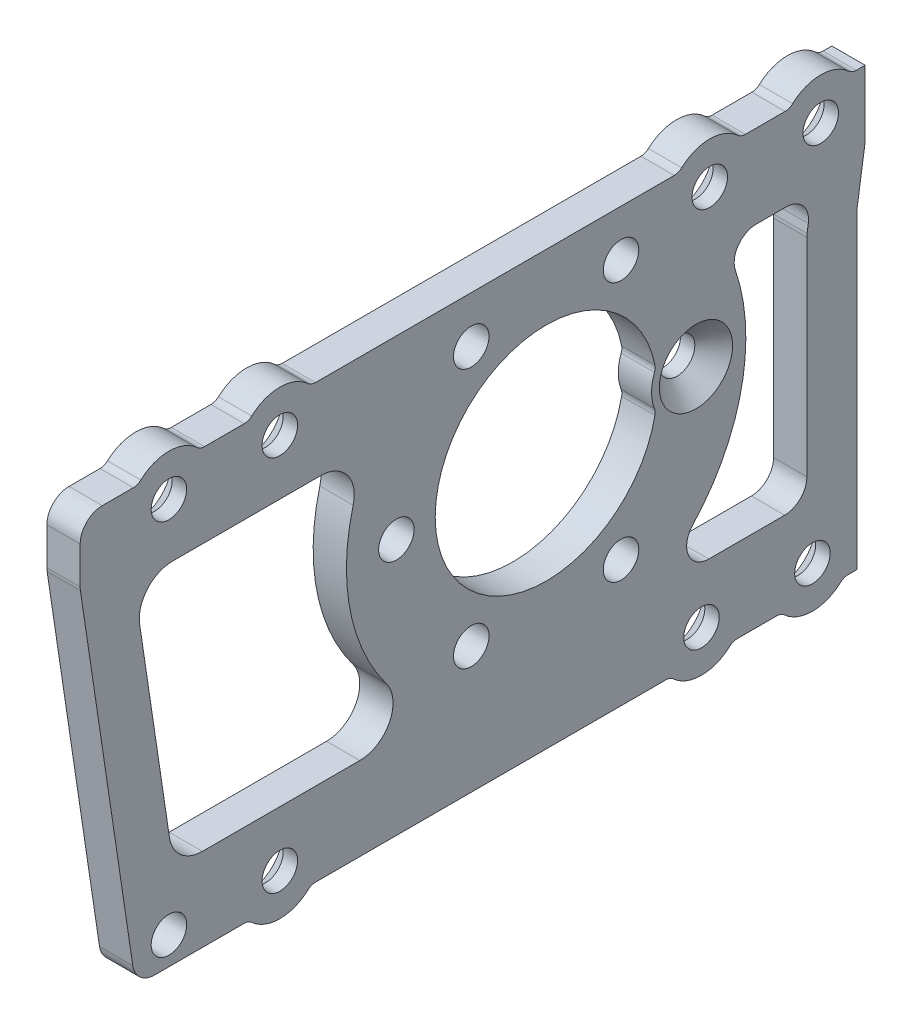
SolidWorks part; units mm, degrees
other "标注1"
sketch "草图13" plane through (3, 17.15, -28.75) normal (0.7677, 0.0888, -0.6346) x (-0.6353, 0.2347, -0.7357)
material "Thornel Mat VMA"
ref_plane "前视基准面" through (0, 0, 0) normal (0, 0, 1) x (1, 0, 0)
ref_plane "上视基准面" through (0, 0, 0) normal (0, 1, 0) x (1, 0, 0)
ref_plane "右视基准面" through (0, 0, 0) normal (1, 0, 0) x (0, 0, -1)
other "Configuration Table"
sketch "草图1" plane through (0, 0, 0) normal (1, 0, 0) x (0, 0, -1)
  line L0 (0, 0) -> (-13.5, 0) construction
  line L4 (0, 0) -> (0, -20.6) construction
  line L6 (28, 4.9) -> (28, -23.1)
  line L7 (28, -23.1) -> (-37, -23.1)
  line L9 (0, -20.6) -> (14, -20.6) construction
  line L10 (14, -20.6) -> (24, -20.6) construction
  line L11 (-51.8773, -23.6) -> (28, -23.6) construction
  line L12 (-55.4482, 16.4) -> (44.8007, 16.4) construction
  line L13 (28, 4.9) -> (28.75, 9.9)
  line L14 (28.75, 9.9) -> (28.75, 15.9)
  line L15 (28.75, 15.9) -> (-42, 15.9)
  line L16 (-42, 15.9) -> (-42, 10.4)
  line L17 (-37, -23.6) -> (-16, -23.6) construction
  line L18 (-37, -23.6) -> (-37, -17.6) construction
  line L19 (-37, -17.6) -> (-16, -17.6) construction
  line L20 (-16, -23.6) -> (-16, -17.6) construction
  line L21 (-42, 10.4) -> (-21, 10.4) construction
  line L22 (-42, 10.4) -> (-42, 16.4) construction
  line L23 (-42, 16.4) -> (-21, 16.4) construction
  line L24 (-21, 10.4) -> (-21, 16.4) construction
  line L25 (-42, 10.4) -> (-37, -23.1)
  circle A0 centre (0, 0) radius 13.5 construction
  circle A1 centre (-13.5, 0) radius 1.6
  circle A2 centre (-6.75, 11.6913) radius 1.6
  circle A3 centre (6.75, 11.6913) radius 1.6
  circle A4 centre (13.5, 0) radius 1.6
  circle A5 centre (6.75, -11.6913) radius 1.6
  circle A6 centre (-6.75, -11.6913) radius 1.6
  circle A7 centre (0, 0) radius 10
  circle A9 centre (14, -20.6) radius 1.6
  circle A10 centre (24, -20.6) radius 1.6
  circle A11 centre (24.75, 13.4) radius 1.6
  circle A12 centre (14.75, 13.4) radius 1.6
  circle A13 centre (0, 0) radius 28.5 construction
  circle A14 centre (-24, -20.6) radius 1.6 construction
  circle A15 centre (-34, -20.6) radius 1.6 construction
  circle A16 centre (-24, -20.6) radius 3 construction
  circle A17 centre (-24, -20.6) radius 1.6
  circle A18 centre (-34, -20.6) radius 1.6
  circle A19 centre (-34, 13.4) radius 1.6
  circle A20 centre (-24, 13.4) radius 1.6
  point P17 (0, 0)
  dimension "D1" = 27
  dimension "D2" = 3.2
  dimension "D4" = 20
  dimension "D5" = 3
  dimension "D10" = 3.2
  dimension "D12" = 3.2
  dimension "D16" = 3.2
  dimension "D17" = 3.2
  dimension "D18" = 10
  dimension "D19" = 8
  dimension "D23" = 57
  dimension "D26" = 3.2
  dimension "D27" = 3.2
  dimension "D28" = 24
  dimension "D29" = 3
  dimension "D30" = 10
  dimension "D32" = 6
  dimension "D33" = 3.2
  dimension "D34" = 3.2
  dimension "D6" = 23.1
  dimension "D7" = 28
  dimension "D8" = 14
  dimension "D9" = 20.6
  dimension "D11" = 10
  dimension "D13" = 4
  dimension "D14" = 0.5
  dimension "D15" = 40
  dimension "D20" = 6
  dimension "D21" = 1
  dimension "D22" = 4
  dimension "D24" = 21
  dimension "D25" = 6
  dimension "D31" = 3
  dimension "D35" = 3
  dimension "D36" = 3
  dimension "D37" = 10
  dimension "D38" = 3
  dimension "D39" = 6
  dimension "D40" = 3
  dimension "D41" = 8
  dimension "D3" = 6
extrude "凸台-拉伸1" add sketch "草图1" along normal blind 3
sketch "草图2" plane through (0, 0, 0) normal (-1, 0, 0) x (0, 0, 1)
  circle A0 centre (-24.75, 13.4) radius 1.6
  circle A1 centre (-24.75, 13.4) radius 3.75
  circle A2 centre (-14.75, 13.4) radius 1.6
  circle A3 centre (-14.75, 13.4) radius 3.75
  circle A4 centre (24, 13.4) radius 1.6
  circle A5 centre (24, 13.4) radius 3.75
  circle A6 centre (24, -20.6) radius 1.6
  circle A7 centre (24, -20.6) radius 3.75
  circle A8 centre (-24, -20.6) radius 1.6
  circle A9 centre (-14, -20.6) radius 1.6
  circle A10 centre (-24, -20.6) radius 3.75
  circle A11 centre (-14, -20.6) radius 3.75
  circle A14 centre (-13.5, 0) radius 1.6
  circle A15 centre (-13.5, 0) radius 4
  circle A16 centre (34, 13.4) radius 3.75
  circle A17 centre (34, 13.4) radius 1.6
  dimension "D1" = 7.5
  dimension "D2" = 3.2
  dimension "D3" = 3.2
  dimension "D4" = 7.5
  dimension "D5" = 3.2
  dimension "D6" = 7.5
  dimension "D7" = 3.2
  dimension "D8" = 7.5
  dimension "D9" = 3.2
  dimension "D10" = 3.2
  dimension "D11" = 7.5
  dimension "D12" = 7.5
  dimension "D13" = 8
  dimension "D14" = 3.2
  dimension "D15" = 7.5
  dimension "D16" = 3.2
extrude "凸台-拉伸2" add sketch "草图2" against normal up to surface (3 mm away) up to face at (3, 13.4, 32.4)
hole_wizard "M3 十字槽半沉头木螺钉的锥形沉头孔1" positions "草图16" profile "草图15" countersink size "M3" standard "GB"
sketch "草图16" plane through (0, 0, 0) normal (-1, 0, 0) x (0, 0, 1)
  point P0 (-24.75, 13.4)
  point P3 (-14.75, 13.4)
  point P6 (-24, -20.6)
  point P9 (-14, -20.6)
  point P12 (24, 13.4)
  point P15 (34, 13.4)
  point P18 (24, -20.6)
sketch "草图15" plane through (0, 13.4, -24.75) normal (0, 1, 0) x (0, 0, 1)
  line L0 (0, 0) -> (0, 8.4614)
  line L1 (0, 8.4614) -> (1.6, 7.5)
  line L2 (1.6, 7.5) -> (1.6, 1.7)
  line L3 (1.6, 1.7) -> (3.3, 0)
  line L5 (3.3, 0) -> (0, 0)
  line L6 (-1.6, 1.7) -> (-3.3, 0) construction
  line L10 (0, 8.4614) -> (-1.6, 7.5) construction
  line L11 (0, -6.35) -> (0, 107.95) construction
  dimension "孔直径" = 3.2
  dimension "孔深度" = 7.5
  dimension "近端锥形沉头孔直径" = 6.6
  dimension "近端锥形沉头孔角度" = 90
  dimension "导头角度" = 118
sketch "草图17" plane through (0, 0, 0) normal (-1, 0, 0) x (0, 0, 1)
  line L0 (15.9198, 8.4) -> (37.1516, 8.4)
  line L1 (37.1516, 8.4) -> (33.5696, -15.6)
  line L2 (33.5696, -15.6) -> (8.98, -15.6)
  line L3 (42, 10.4) -> (37, -23.1) construction
  line L4 (-11.9549, 15.9) -> (21.2049, 15.9) construction
  line L5 (21.2049, -23.1) -> (-11.2049, -23.1) construction
  line L6 (-15.9198, 8.4) -> (-23.9747, 8.4)
  line L7 (-23.9747, 8.4) -> (-23.5, 5.2356)
  line L8 (-23.5, -15.6) -> (-8.98, -15.6)
  line L9 (-28, 4.9) -> (-28.75, 9.9) construction
  line L10 (-23.5, 5.2356) -> (-23.5, -15.6)
  line L11 (-28, -23.1) -> (-28, 4.9) construction
  circle A0 centre (0, 0) radius 18
  circle A1 centre (13.5, 0) radius 3.5 construction
  dimension "D1" = 36
  dimension "D2" = 7
  dimension "D3" = 7.5
  dimension "D4" = 7.5
  dimension "D5" = 4.5
  dimension "D6" = 4.5
  dimension "D7" = 4.5
extrude "切除-拉伸1" cut sketch "草图17" against normal blind 10 contours A0 L2 L1 L0 | A0 L6 L7 L10 L8
hole_wizard "M3 十字槽半沉头木螺钉的锥形沉头孔2" positions "草图20" profile "草图19" countersink size "M3" standard "GB"
sketch "草图20" plane through (3, 0, 0) normal (1, 0, 0) x (0, 0, -1)
  point P0 (13.5, 0)
sketch "草图19" plane through (3, 0, -13.5) normal (0, 1, 0) x (0, 0, -1)
  line L0 (0, 0) -> (0, 8.4614)
  line L1 (0, 8.4614) -> (1.6, 7.5)
  line L2 (1.6, 7.5) -> (1.6, 1.7)
  line L3 (1.6, 1.7) -> (3.3, 0)
  line L5 (3.3, 0) -> (0, 0)
  line L6 (-1.6, 1.7) -> (-3.3, 0) construction
  line L10 (0, 8.4614) -> (-1.6, 7.5) construction
  line L11 (0, -6.35) -> (0, 107.95) construction
  dimension "孔直径" = 3.2
  dimension "孔深度" = 7.5
  dimension "近端锥形沉头孔直径" = 6.6
  dimension "近端锥形沉头孔角度" = 90
  dimension "导头角度" = 118
fillet "圆角1" radius 3 4 edges at (1.5, -15.6, 33.5696) (1.5, 8.4, 37.1516) (1.5, -15.6, 8.98) (1.5, 8.4, 15.9198)
fillet "圆角2" radius 2 10 edges at (1.5, -23.1, 37) (1.5, 15.9, 42) (1.5, 10.4, 42) (1.5, 9.9, -28.75) (1.5, 4.9, -28) (1.5, -15.6, -23.5) (1.5, 5.2356, -23.5) (1.5, 8.4, -15.9198) (1.5, -15.6, -8.98) (1.5, 8.4, -23.9747)
fillet "圆角3" radius 1 16 edges at (1.5, -23.1, -16.7951) (1.5, -23.1, -11.2049) (1.5, -23.1, -26.7951) (1.5, -23.1, -21.2049) (1.5, -23.1, 21.2049) (1.5, -23.1, 26.7951) (1.5, 15.9, 36.7951) (1.5, 15.9, 31.2049) (1.5, 15.9, 26.7951) (1.5, 15.9, 21.2049) (1.5, 15.9, -11.9549) (1.5, 15.9, -17.5451) (1.5, 15.9, -21.9549) (1.5, 15.9, -27.5451) (1.5, -1.6609, -9.8611) (1.5, 1.6609, -9.8611)
